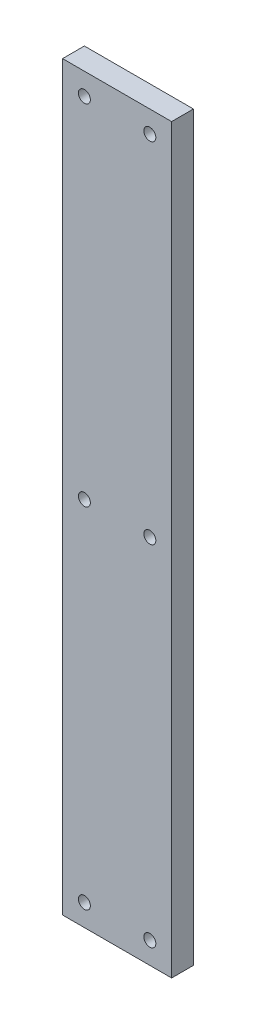
SolidWorks part; units mm, degrees
material "Rubber"
ref_plane "Front Plane" through (0, 0, 0) normal (0, 0, 1) x (1, 0, 0)
ref_plane "Top Plane" through (0, 0, 0) normal (0, 1, 0) x (1, 0, 0)
ref_plane "Right Plane" through (0, 0, 0) normal (1, 0, 0) x (0, 0, -1)
sketch "Sketch1" plane through (0, 0, 0) normal (0, 0, 1) x (1, 0, 0)
  line L1 (0, 0) -> (100, 0)
  line L2 (0, 0) -> (0, -680)
  line L3 (0, -680) -> (100, -680)
  line L4 (100, 0) -> (100, -680)
  dimension "D1" = 100
  dimension "D2" = 680
extrude "Boss-Extrude1" add sketch "Sketch1" along normal blind 20
sketch "Sketch2" plane through (0, 0, 20) normal (0, 0, 1) x (1, 0, 0)
  line L0 (100, 0) -> (0, 0) construction
  line L1 (0, 0) -> (0, -680) construction
  circle A0 centre (20, -20) radius 5.5
  dimension "D3" = 11
  dimension "D1" = 20
  dimension "D2" = 20
extrude "Cut-Extrude1" cut sketch "Sketch2" against normal blind 20
pattern_linear "LPattern1" count 2 spacing 60 along (1, 0, 0) count 3 spacing 320 along (0, -1, 0) of "Cut-Extrude1"
